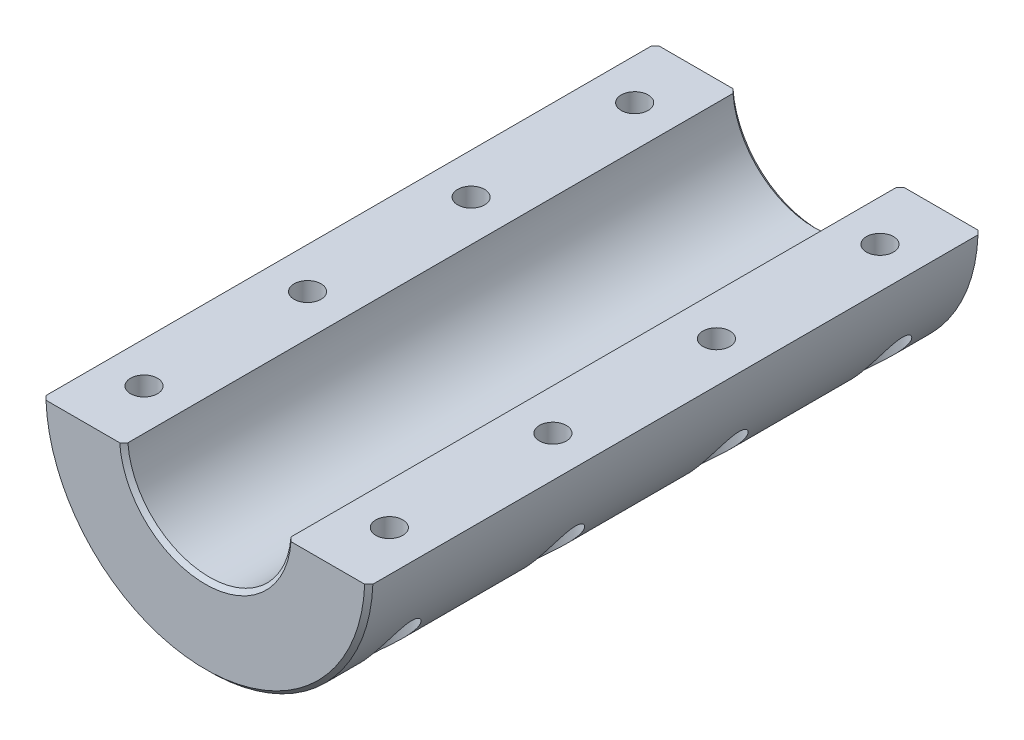
from build123d import *

# Parameters (mm, degrees)
SKETCH1_R            = 40
BOSS_EXTRUDE1_DEPTH  = 75
CHAMFER1_SIZE        = 1
SKETCH2_W            = 85
SKETCH2_H            = 3
CUT_EXTRUDE1_DEPTH   = 180
CUT_EXTRUDE2_START   = -9
SKETCH6_R            = 5.5
CUT_EXTRUDE2_DEPTH   = 91
LPATTERN1_COUNT      = 4
LPATTERN1_PITCH      = 40
LPATTERN1_COUNT_DIR2 = 2
LPATTERN1_PITCH_DIR2 = 60


with BuildPart() as part:
    # Sketch1 → Boss-Extrude1 (new, symmetric)
    with BuildSketch(Plane.XY):
        Circle(SKETCH1_R)
        with BuildLine():
            Line((-4, 15.3), (4, 15.3))
            Line((4, 15.3), (4, 19.595917942))
            ThreePointArc((4, 19.595917942), (0, -20), (-4, 19.595917942))
            Line((-4, 19.595917942), (-4, 15.3))
        make_face(mode=Mode.SUBTRACT)
    extrude(amount=BOSS_EXTRUDE1_DEPTH, both=True)

    # Chamfer1
    chamfer1_edges = [part.edges().sort_by_distance(p)[0] for p in [
        (-40, 0, -75),
        (-40, 0, 75),
        (0, -20, -75),
        (0, -20, 75),
    ]]
    chamfer(chamfer1_edges, length=CHAMFER1_SIZE)

    # Sketch2 → Cut-Extrude1 (cut)
    with BuildSketch(Plane.XY.offset(75)):
        Rectangle(SKETCH2_W, SKETCH2_H)
    extrude(amount=-CUT_EXTRUDE1_DEPTH, mode=Mode.SUBTRACT)


with BuildPart() as cut_extrude1_kept_piece:
    # of the separate pieces the step leaves, the one the design keeps (cut_extrude1_pieces_kept)
    add(part.part.solids().sort_by_distance((-39.971865105, -1.5, -74))[0])

    # Sketch5 → M6 Clearance Hole1 (revolve, cut)
    with BuildSketch(Plane(origin=(30, -1.5, 60), x_dir=(0, 0, 1), z_dir=(1, 0, 0))):
        Polygon((0, 0), (0, 36.982840043), (3.3, 35), (3.3, 0), align=None)
    m6_clearance_hole1 = revolve(axis=Axis((30, 4.85, 60), (0, -1, 0)), mode=Mode.SUBTRACT)

    # Sketch6 → Cut-Extrude2 (cut)
    with BuildSketch(Plane(origin=(0, -1.5, 0), x_dir=(1, 0, 0), z_dir=(0, 1, 0)).offset(CUT_EXTRUDE2_START)):
        with Locations(Location((30, -60, 0), (0, 0, 270))):
            Circle(SKETCH6_R)
    cut_extrude2 = extrude(amount=-CUT_EXTRUDE2_DEPTH, mode=Mode.SUBTRACT)

    # LPattern1: M6 Clearance Hole1, Cut-Extrude2 4 × 2
    with Locations(*[(-j * LPATTERN1_PITCH_DIR2, 0, -i * LPATTERN1_PITCH) for i in range(LPATTERN1_COUNT) for j in range(LPATTERN1_COUNT_DIR2) if (i, j) != (0, 0)]):
        add(m6_clearance_hole1, mode=Mode.SUBTRACT)
        add(cut_extrude2, mode=Mode.SUBTRACT)


solid = cut_extrude1_kept_piece.part
